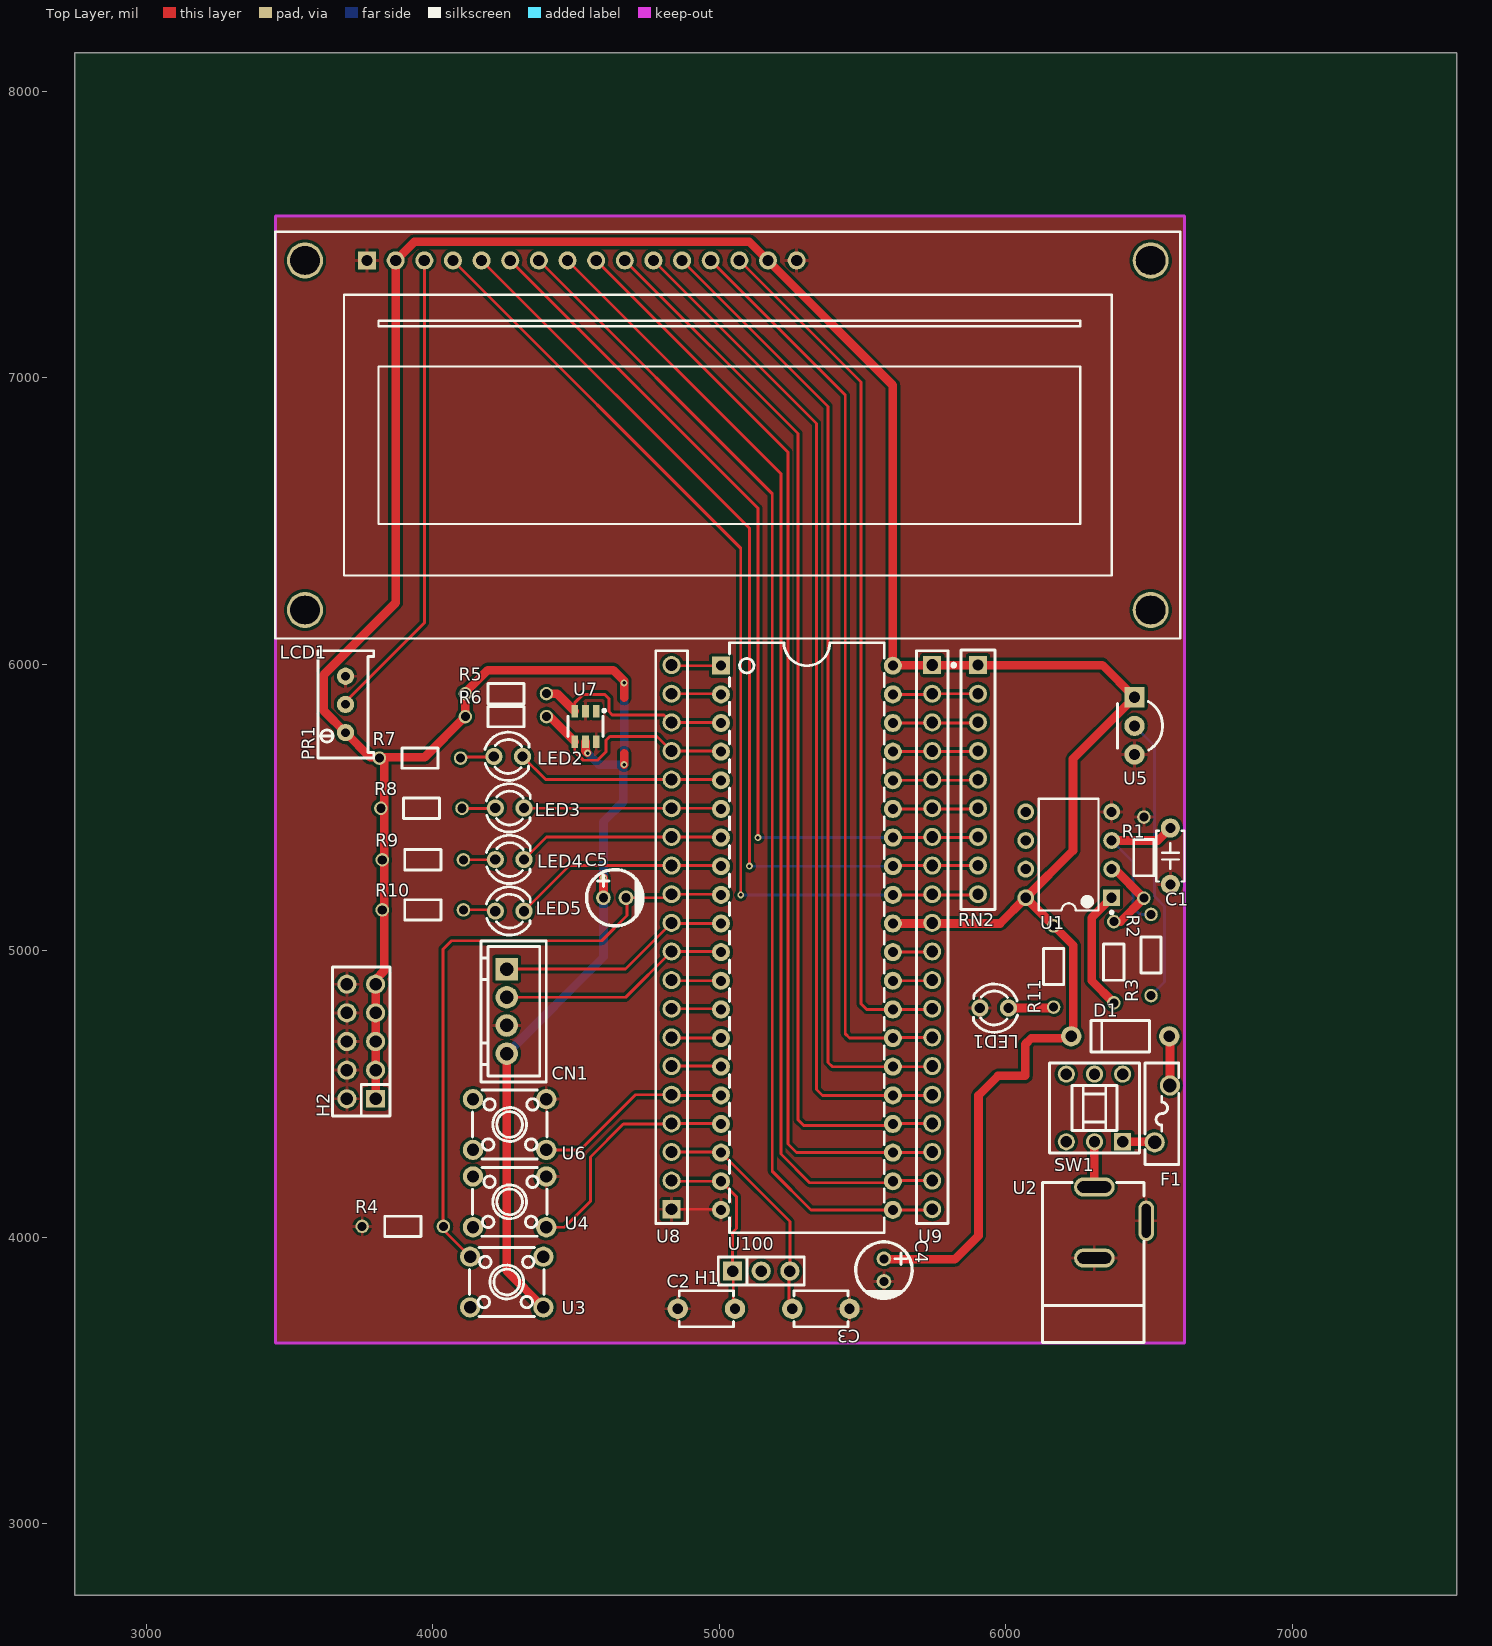
[diagram p0: Top Layer view]
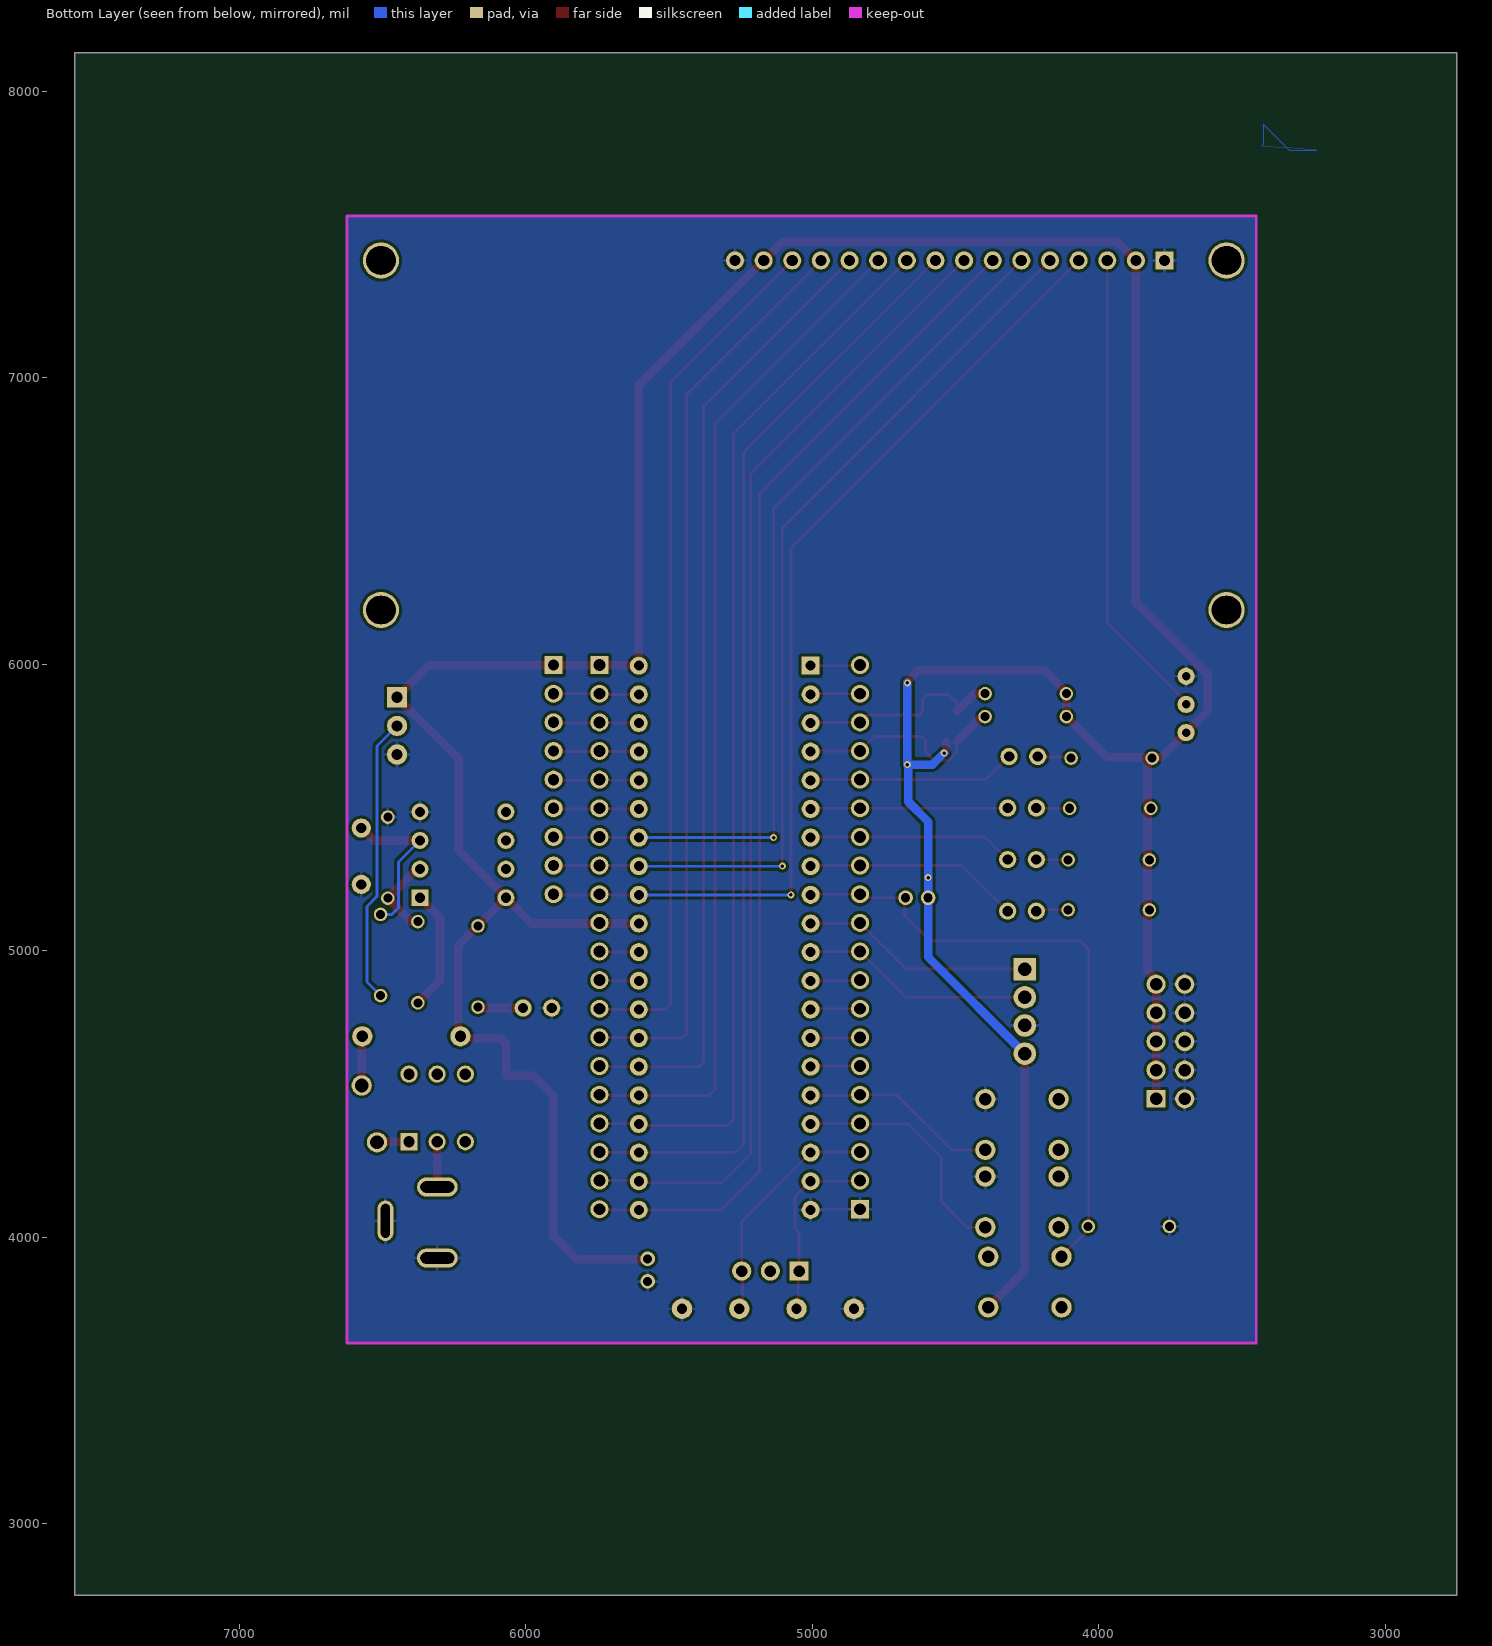
[diagram p1: Bottom Layer view, seen from below]
# Altium PCB MISC75226.pcbdoc
Units mil, origin at the board's own origin, x right, y up, seen from the top; angles counter-clockwise.
Board outline 4825 x 5385 mil, 2 copper layers (Top Layer, Bottom Layer), stack 2.757 mil thick; 40 components, 54 nets, 213 pads, 7 vias.

## Layer stack, top to bottom
Top Solder Mask Layer: solder mask 0.394, Dk 3.3
Top Layer: signal copper 1.379
Bottom Layer: signal copper 1.378
Bottom Solder Mask Layer: solder mask 0.394, Dk 3.3

## Board outline
7575,2750 2750,2750 2750,8135 7575,8135

## Design rules (kind name [scope] priority, off if disabled: settings)
BoardOutlineClearance Default_1 [All] p2: genericclearance=4 ignorepadtopadclearanceinfootprint=FALSE except(0: Arc-SplitContinuation Track-SplitContinuation SMDPad-SplitContinuation THPad-SplitContinuation Via-SplitContinuation Fill-SplitContinuation Region-SplitContinuation Poly-SplitContinuation Text-SplitContinuation Hole-SplitContinuation; 6: Arc-OutlineEdge Track-OutlineEdge SMDPad-OutlineEdge THPad-OutlineEdge Via-OutlineEdge Fill-OutlineEdge Region-OutlineEdge Poly-OutlineEdge Text-OutlineEdge Hole-OutlineEdge SMDPad-CutoutEdge THPad-CutoutEdge Via-CutoutEdge Fill-CutoutEdge Region-CutoutEdge Text-CutoutEdge; 6.9: Hole-CutoutEdge; 10: Poly-CutoutEdge; 11.8: Arc-CutoutEdge Track-CutoutEdge)
Clearance Default [All] p1: gap=4 ignorepadtopadclearanceinfootprint=FALSE except(6: SMDPad-Track SMDPad-SMDPad THPad-Track SMDPad-THPad THPad-THPad Track-Via SMDPad-Via THPad-Via Via-Via Fill-Track Region-Track Fill-SMDPad Region-SMDPad Fill-THPad Region-THPad Fill-Via Region-Via Fill-Fill Fill-Region Region-Region Arc-Track Arc-SMDPad Arc-THPad Arc-Via Fill-Arc Region-Arc Arc-Arc Text-Track SMDPad-Text Text-THPad Text-Via Fill-Text Region-Text Arc-Text Text-Text; 6.9: Hole-Track Hole-SMDPad Hole-THPad Hole-Via Fill-Hole Region-Hole Hole-Arc Hole-Text; 10: Poly-Track Poly-SMDPad Poly-THPad Poly-Via Poly-Fill Poly-Region Poly-Poly Poly-Arc Poly-Text Poly-Hole)
DiffPairsRouting differentialPair [All] p1: maxlimit=6 minlimit=5 mostfreqgap=6 toplayer_minwidth=5 toplayer_prefwidth=100 toplayer_maxwidth=100 toplayer_mingap=5 toplayer_prefgap=6 toplayer_maxgap=6 bottomlayer_minwidth=5 bottomlayer_prefwidth=100 bottomlayer_maxwidth=100 bottomlayer_mingap=5 bottomlayer_prefgap=6 bottomlayer_maxgap=6 maxuncoupledlength=10
HoleToHoleClearance otherClearance [All] p1: gap=11.8 allowstackedmicrovias=TRUE
Length netLength [All] p1: minlimit=0 maxlimit=0
MatchedLengths netLengthTolerance [All] p1: tolerance=1000
PasteMaskExpansion pasteMaskExpansion [All] p1: expansion=0
PlaneConnect innerPlane [All] p1: planeconnectstyle=Relief reliefexpansion=20 reliefentries=4 reliefconductorwidth=10 reliefairgap=10
PolygonConnect copperRegion [All] p1: connectstyle=Relief reliefconductorwidth=10 reliefentries=4 polygonreliefangle="90 Angle" airgapwidth=10 via.connectstyle=Relief via.reliefconductorwidth=10 via.reliefentries=4 via.polygonreliefangle="90 Angle" via.airgapwidth=10
RoutingVias Default_3 [All] p1: holewidth=12 width=24 viastyle="Through Hole" minholewidth=12 minwidth=24 maxholewidth=1181 maxwidth=1969
SolderMaskExpansion Common [IsVia] p1: expansion=-1000 istentingtop=TRUE
SolderMaskExpansion Common [All] p2: expansion=2 istentingtop=FALSE
Width Default_2 [All] p1: maxlimit=1000 minlimit=10 preferedwidth=10

## Components (designator, comment, footprint, x,y, rotation, side; value= is the part's Value field where it differs from the comment)
C1 "10nF" CAP-TH_L4.5-W2.5-P5.00-D0.5 6575,5330 r90 top
C2 "22pF" CAP-TH_L4.8-W3.2-P5.08-D0.5 4955,3750 r0 top
C3 "22pF" CAP-TH_L4.8-W3.2-P5.08-D0.5 5355,3750 r180 top
C4 "10uF" CAP-TH_BD5.0-P2.00-D0.8-FD-10UF50VC110GL 5575,3885 r270 top
C5 "10uF" CAP-TH_BD5.0-P2.00-D0.8-FD-10UF50VC110GL 4635,5185 r0 top
CN1 "HEADER 4" CONN-TH_XH-4A 4258.04,4788.24 r270 top
D1 "1N4007" DO-41_BD2.4-L4.7-P8.70-D0.9-RD 6400.04,4701.07 r0 top
F1 "JK60-050" FUSE-TH_L8.9-W3.0-P5.10-D0.6-S1.20 6545.04,4431.07 r90 top
H1 "PZ254V-11-03P_C2937625" HDR-TH_3P-P2.54-V-M_PZ254V-11-03P 5146.55,3881.61 r0 top
H2 "" HDR-TH_10P-P2.54-V-F-R2-C5-S2.54 3749.9,4683.05 r90 top
LCD1 "HS1602A" LCD1602 5030,6800 r0 top
LED1 "" LED_TH-3mm 5960,4800 r180 top
LED2 "HL-304S9AD" LED-TH_BD3.0-P2.54-FD 4263.04,5678.24 r0 top
LED3 "HL-304S9AD" LED-TH_BD3.0-P2.54-FD 4268.04,5498.24 r0 top
LED4 "HL-304S9AD" LED-TH_BD3.0-P2.54-FD 4268.04,5318.24 r0 top
LED5 "HL-304S9AD" LED-TH_BD3.0-P2.54-FD 4268.04,5138.24 r0 top
PR1 "10kΩ" R_3296 3690,5860 r90 top
R1 "10kΩ" Res_1/8W 6480,5325 r270 top
R2 "10kΩ" Res_1/8W 6375,4960 r270 top
R3 "10kΩ" Res_1/8W 6510,4985 r90 top
R4 "10kΩ" Res_1/8W 3895,4035 r0 top
R5 "10kΩ" Res_1/8W 4255,5895 r0 top
R6 "10kΩ" Res_1/8W 4255,5815 r0 top
R7 "1kΩ" Res_1/8W 3955,5670 r0 top
R8 "1kΩ" Res_1/8W 3960,5495 r0 top
R9 "1kΩ" Res_1/8W 3965,5315 r0 top
R10 "1kΩ" Res_1/8W 3965,5140 r0 top
R11 "1kΩ" Res_1/8W 6170,4945 r90 top
RN2 "10K" RES-ARRAY-TH_9P-P2.54-D1.0 5903.48,5597.32 r270 top
SW1 "HX 8-8 ZS" SW-TH_6P-L8.0-W8.0-P2.50-TL 6310.04,4451.07 r180 top
U1 "LM358AN" DIP-8_L9.8-W6.6-P2.54-LS7.6-BL 6220,5335 r90 top
U2 "DC005-2.5" DC-IN-TH_DC005-2.5MM 6400.04,4051.07 r90 top
U3 "TC-00104FS-075E" KEY-TH_4P-L6.0-W6.0-P4.50-LS6.5 4258.04,3843.24 r0 top
U4 "TC-00104FS-075E" KEY-TH_4P-L6.0-W6.0-P4.50-LS6.5 4268.04,4123.24 r180 top
U5 "LM35DZ/NOPB" TO-92-3_L4.8-W3.7-P2.54-L 6450,5785 r270 top
U6 "TC-00104FS-075E" KEY-TH_4P-L6.0-W6.0-P4.50-LS6.5 4268.04,4393.24 r180 top
U7 "ADS1110A1IDBVR" SOT-23-6_L2.9-W1.6-P0.95-LS2.8-BR 4533.04,5783.24 r90 top
U8 "[Plugin] 2.54MM 1*20P straight female header-H5.0" HDR-TH_20P-P2.54_C9900009338 4833.48,5047.32 r90 top
U9 "[Plugin] 2.54MM 1*20P straight female header-H5.0" HDR-TH_20P-P2.54_C9900009338 5743.48,5047.32 r270 top
U100 "STC89C52RC-40I" DIP-40_L52.0-W13.7-P2.54-LS15.2-BL 5305.96,5045.14 r270 top

## Footprints (in the part's own frame and the unit in brackets; to place one, negate y for a bottom-side part, rotate by r counter-clockwise, add the part's x,y. Pads: shape width x height; smd on the part's side, far side on the other; paste and mask are expansions set on the pad)
CAP-TH_BD5.0-P2.00-D0.8-FD-10UF50VC110GL [mm]
  round 1.3 hole 0.8: 1(-1,0) 2(1,0)
  silkscreen extent -2.5,-2.5 2.5,2.5
CAP-TH_L4.5-W2.5-P5.00-D0.5 [mm]
  round 1.7 hole 0.9 paste+0 mask+0.05: 1(-2.5,0) 2(2.5,0)
  silkscreen extent -2.25,-1.25 2.25,1.25
CAP-TH_L4.8-W3.2-P5.08-D0.5 [mm]
  round 1.8 hole 0.9: 1(-2.54,0) 2(2.54,0)
  silkscreen extent -2.4,-1.6 2.4,1.6
CONN-TH_XH-4A [mm]
  rect 2x2 hole 1.2 paste+0 mask+0.051: 1(-3.75,0)
  round 2 hole 1.2 paste+0 mask+0.051: 2(-1.25,0) 3(1.25,0) 4(3.75,0)
  silkscreen extent -6.25,-2.3 6.25,3.5
DC-IN-TH_DC005-2.5MM [mm]
  oval 3.6x1.4 hole 0.8 slot 3 at 0 deg copper offset 0,0 paste+0 mask+0.05: 2(0.15,-2.3)
  oval 1.7x3.6 hole 1 slot 3 at 90 deg copper offset 0,0 paste+0 mask+0.05: 3(-3.15,2.3)
  oval 1.7x3.6 hole 1 slot 3 at 90 deg paste+0 mask+0.05: 4(3.15,2.3)
  silkscreen extent -10.65,-2.1 3.55,6.9
DIP-8_L9.8-W6.6-P2.54-LS7.6-BL [mm]
  rect 1.5x1.5 hole 0.9 paste+0 mask+0.051: 1(-3.81,-3.81)
  round 1.5 hole 0.9 paste+0 mask+0.051: 2(-1.27,-3.81) 3(1.27,-3.81) 4(3.81,-3.81) 5(3.81,3.81) 6(1.27,3.81) 7(-1.27,3.81) 8(-3.81,3.81)
  silkscreen extent -5.23,-3.93 4.96,2.65
DIP-40_L52.0-W13.7-P2.54-LS15.2-BL [mil]
  rect 63x63 hole 35 paste+0 mask+2: 1(-950,-300)
  round 63 hole 35 paste+0 mask+2: 2(-850,-300) 3(-750,-300) 4(-650,-300) 5(-550,-300) 6(-450,-300) 7(-350,-300) 8(-250,-300) 9(-150,-300) 10(-50,-300) 11(50,-300) 12(150,-300) 13(250,-300) 14(350,-300) 15(450,-300) 16(550,-300) 17(650,-300) 18(750,-300) 19(850,-300) 20(950,-300) 21(950,300) 22(850,300) 23(750,300) 24(650,300) 25(550,300) 26(450,300) 27(350,300) 28(250,300) 29(150,300) 30(50,300) 31(-50,300) 32(-150,300) 33(-250,300) 34(-350,300) 35(-450,300) 36(-550,300) 37(-650,300) 38(-750,300) 39(-850,300) 40(-950,300)
  silkscreen extent -1030,-270 1030,270
DO-41_BD2.4-L4.7-P8.70-D0.9-RD [mm]
  round 1.8 hole 1 paste+0 mask+0.051: 1(-4.35,0) 2(4.35,0)
  silkscreen extent -2.6,-1.4 2.6,1.4
FUSE-TH_L8.9-W3.0-P5.10-D0.6-S1.20 [mm]
  round 1.8 hole 1.2 paste+0 mask+0.051: 1(-2.54,0.635) 2(2.499,-0.727)
  silkscreen extent -4.5,-1.5 4.5,1.5
HDR-TH_3P-P2.54-V-M_PZ254V-11-03P [mm]
  rect 1.7x1.7 hole 1.02 paste+0 mask+0.051: 1(-2.54,0)
  round 1.7 hole 1.02 paste+0 mask+0.051: 2(0,0) 3(2.54,0)
  silkscreen extent -3.81,-1.25 3.81,1.25
HDR-TH_10P-P2.54-V-F-R2-C5-S2.54 [mm]
  rect 1.575x1.7 hole 1.1: 1(-5.08,-1.27)
  round 1.7 hole 1.1: 2(-5.08,1.27) 3(-2.54,-1.27) 4(-2.54,1.27) 5(0,-1.27) 6(0,1.27) 7(2.54,-1.27) 8(2.54,1.27) 9(5.08,-1.27) 10(5.08,1.27)
  silkscreen extent -6.6,-2.54 6.6,2.54
HDR-TH_20P-P2.54_C9900009338 [mm]
  rect 1.6x1.6 hole 1.05 paste+0 mask+0.051: 1(-24.13,0)
  round 1.6 hole 1.05 paste+0 mask+0.051: 2(-21.59,0) 3(-19.05,0) 4(-16.51,0) 5(-13.97,0) 6(-11.43,0) 7(-8.89,0) 8(-6.35,0) 9(-3.81,0) 10(-1.27,0) 11(1.27,0) 12(3.81,0) 13(6.35,0) 14(8.89,0) 15(11.43,0) 16(13.97,0) 17(16.51,0) 18(19.05,0) 19(21.59,0) 20(24.13,0)
  silkscreen extent -25.4,-1.4 25.4,1.4
KEY-TH_4P-L6.0-W6.0-P4.50-LS6.5 [mm]
  round 1.8 hole 1.1 paste+0 mask+0.051: 1(-3.251,-2.25) 2(3.251,-2.25) 3(3.251,2.25) 4(-3.251,2.25)
  silkscreen extent -3.3,-3.05 3.3,3.05
LCD1602 [mm]
  round 3.2 hole 2.5 slot 2.625 at 0 deg paste+0 mask+0.051: 0(-37.5,-15.5) 0(-37.5,15.5) 0(37.5,-15.5) 0(37.5,15.5)
  rect 1.6x1.6 hole 1 paste+0 mask+0.051: 1(-32,15.5)
  round 1.6 hole 1 paste+0 mask+0.051: 2(-29.46,15.5) 3(-26.92,15.5) 4(-24.38,15.5) 5(-21.84,15.5) 6(-19.3,15.5) 7(-16.76,15.5) 8(-14.22,15.5) 9(-11.68,15.5) 10(-9.14,15.5) 11(-6.6,15.5) 12(-4.06,15.5) 13(-1.52,15.5) 14(1.02,15.5) 15(3.56,15.5) 16(6.1,15.5)
  silkscreen extent -40.13,-18.03 40.13,18.03
LED-TH_BD3.0-P2.54-FD [mil]
  round 60 hole 36 paste+0 mask+1.97: 1(-50,0) 2(50,0)
  silkscreen extent -81,-84 72,85
LED_TH-3mm [mil]
  round 60 hole 36 paste+0 mask+2: 1(-50,0) 2(50,0)
  silkscreen extent -81,-84 72,85
R_3296 [mil]
  round 60 hole 30 paste+0 mask+2: 1(-98.4,-5) 2(0,-5) 3(98.4,-5)
  silkscreen extent -187,-103 187,92
RES-ARRAY-TH_9P-P2.54-D1.0 [mm]
  rect 1.6x1.6 hole 1 paste+0 mask+0.051: 1(-10.16,0)
  round 1.6 hole 1 paste+0 mask+0.051: 2(-7.62,0) 3(-5.08,0) 4(-2.54,0) 5(0,0) 6(2.54,0) 7(5.08,0) 8(7.62,0) 9(10.16,0)
  silkscreen extent -11.5,-2.31 11.5,1.5
Res_1/8W [mil]
  round 47.2 hole 31.5 paste+0 mask+2: 1(-141.7,2.48) 2(141.7,2.48)
  silkscreen extent -63,-33 63,38
SOT-23-6_L2.9-W1.6-P0.95-LS2.8-BR [mm]
  rect 1.1x0.6 smd paste+0 mask+0.051: 1(1.35,-0.95) 2(1.35,0) 3(1.35,0.95) 4(-1.35,0.95) 5(-1.35,0) 6(-1.35,-0.95)
  silkscreen extent -0.9,-1.78 1.52,1.55
SW-TH_6P-L8.0-W8.0-P2.50-TL [mil]
  rect 60x60 hole 39.37 paste+0 mask+2: 1(-98.42,118.11)
  round 60 hole 39.37 paste+0 mask+2: 2(0.01,118.11) 3(98.43,118.11) 4(-98.42,-118.11) 5(0.01,-118.11) 6(98.43,-118.11)
  silkscreen extent -157,-157 157,157
TO-92-3_L4.8-W3.7-P2.54-L [mm]
  rect 1.8x1.8 hole 1 paste+0 mask+0.051: 1(-2.54,0)
  round 1.8 hole 1 paste+0 mask+0.051: 2(0,0) 3(2.54,0)
  silkscreen extent -2.17,-1.5 2.14,2.48

## Via types
v1: diameter 24.41, hole 12.2, Top Layer to Bottom Layer, 7 vias

## Nets (pads, with @x,y where several pads share a name; then routed paths per layer and width w, separated by ;. In a path a pad name is that pad's centre, name@x,y a point inside that pad or via, vN(x,y) a via of type N, cw(c..) or ccw(c..) an arc to the next point about the centre after c; other vN are vias at no path point)
$2N1: SW1.2 U2.4 | length 157.9
  Top Layer w30: U2.4 SW1.2
$2N3: F1.1 SW1.1 | length 112.4
  Top Layer w30: SW1.1 6518.15,4332.96 F1.1
$2N4: D1.2 F1.2 | length 176.1
  Top Layer w10: F1.2@6568.66,4529.47 F1.2@6571.16,4531.97
  Top Layer w30: D1.2 6573.66,4698.71 F1.2
$2N6: LED1.1 R11.1 | length 158.9
  Top Layer w30: LED1.1 6164.22,4800 R11.1
$2N21: H1.2
$2N22: C1.2 R3.2 U1.3 | length 561.2
  Top Layer w30: U1.3 6531.57,5385 C1.2
  Bottom Layer w10: U1.3 6445,5310 6445,5150 6468.3,5126.7 R3.2
$2N23: R1.2 R2.1 U1.2 | length 293.4
  Top Layer w30: U1.2 6380.78,5285 R1.2 6400.88,5101.7 R2.1
$2N29: LED2.1 R7.2 | length 111.3
  Top Layer w10: R7.2@4102.7,5675.89 4210.69,5675.89 LED2.1
$2N31: LED3.1 R8.2 | length 116
  Top Layer w10: R8.2@4102.7,5496.68 4216.48,5496.68 LED3.1
$2N32: LED4.1 R9.2 | length 115.3
  Top Layer w10: R9.2@4102.7,5317.5 LED4.1
$2N33: LED5.1 R10.2 | length 117.4
  Top Layer w10: R10.2@4102.7,5143.24 4213.04,5143.24 LED5.1
ALE: U9.11 U100.30 | length 138.4
  Top Layer w10: U100.30 5741.3,4995.14 U9.11
GND: C1.1 C2.1 C3.1 C4.2 CN1.3 H2.2 H2.4 H2.6 H2.8 H2.10 LCD1.1 LCD1.16 LED1.2 PR1.3 R1.1 R4.1 U1.4 U2.2 U2.3 U4.1 U5.3 U6.1 U7.2 U7.6 U8.1 U100.20 | length 173.4
  Top Layer w10: U8.1 5003.78,4097.32 U100.20
P0.0: RN2.2 U9.2 U100.39 | length 298.4
  Top Layer w10: U100.39 5741.3,5895.14 U9.2 RN2.2
P0.1: RN2.3 U9.3 U100.38 | length 298.4
  Top Layer w10: U100.38 5901.3,5795.14 RN2.3
P0.2: RN2.4 U9.4 U100.37 | length 298.4
  Top Layer w10: U100.37 5901.3,5695.14 RN2.4
P0.3: RN2.5 U9.5 U100.36 | length 298.4
  Top Layer w10: U100.36 5901.3,5595.14 RN2.5
P0.4: RN2.6 U9.6 U100.35 | length 298.4
  Top Layer w10: U100.35 5901.3,5495.14 RN2.6
P0.5: LCD1.6 RN2.7 U9.7 U100.34 | length 3142.9
  Top Layer w10: LCD1.6 4270.16,7409.84 5065,6615 5135,6545 v1(5135,5395) ; U100.34 5901.3,5395.14 RN2.7
  Bottom Layer w10: v1(5135,5395) U100.34
P0.6: LCD1.5 RN2.8 U9.8 U100.33 | length 3301.7
  Top Layer w10: LCD1.5 5105,6475.4 v1(5105,5295.14) ; U100.33 5608.14,5297.32 U9.8 RN2.8
  Bottom Layer w10: v1(5105,5295.14) U100.33
P0.7: LCD1.4 RN2.9 U9.9 U100.32 | length 3460.7
  Top Layer w10: LCD1.4 5075,6405.4 v1(5075,5195.14) ; U100.32 5901.3,5195.14 RN2.9
  Bottom Layer w10: v1(5075,5195.14) U100.32
P1.0: U8.20 U100.1 | length 173.4
  Top Layer w10: U8.20 4835.66,5995.14 U100.1
P1.1: U8.19 U100.2 | length 173.4
  Top Layer w10: U8.19 5003.78,5897.32 U100.2
P1.2: R5.2 U7.3 U8.18 U100.3 | length 743.7
  Top Layer w10: U7.3 4495.64,5865.64 4525,5895 4600,5895 4615,5880 4615,5835 4626.42,5823.58 4807.22,5823.58 U8.18 5003.78,5797.32 U100.3
  Top Layer w30: R5.2 4434.55,5897.48 U7.3
P1.3: R6.2 U7.4 U8.17 U100.4 | length 773
  Top Layer w10: U7.4 4495.64,5694.36 4525,5665 4575,5665 4605,5695 4605,5735 4617.9,5747.9 4782.9,5747.9 U8.17 5003.78,5697.32 U100.4
  Top Layer w30: R6.2 4408.25,5817.48 U7.4
P1.4: LED2.2 U8.16 U100.5 | length 727.3
  Top Layer w10: LED2.2 4393.96,5597.32 U8.16 5003.78,5597.32 U100.5
P1.5: LED3.2 U8.15 U100.6 | length 688.9
  Top Layer w10: LED3.2 U8.15 5003.78,5497.32 U100.6
P1.6: LED4.2 U8.14 U100.7 | length 721.6
  Top Layer w10: LED4.2 4397.12,5397.32 U8.14 5003.78,5397.32 U100.7
P1.7: LED5.2 U8.13 U100.8 | length 754.7
  Top Layer w10: LED5.2 4477.12,5297.32 U8.13 5003.78,5297.32 U100.8
P2.0: LCD1.7 U9.20 U100.21 | length 4133
  Top Layer w10: LCD1.7 5185,6595.4 5185,4230 5319.9,4095.1 U100.21 ; U100.21 5741.3,4095.14 U9.20
P2.1: LCD1.8 U9.19 U100.22 | length 4001.6
  Top Layer w10: LCD1.8 5215,6665.4 5215,4290 5315,4190 5600.8,4190 U100.22 ; U100.22 5608.14,4197.32 U9.19
P2.2: LCD1.9 U9.18 U100.23 | length 3879.4
  Top Layer w10: LCD1.9 5240,6740.4 5240,4325 5269.9,4295.1 U100.23 ; U100.23 5741.3,4295.14 U9.18
P2.3: LCD1.10 U9.17 U100.24 | length 3730.5
  Top Layer w10: LCD1.10 5275,6805.4 5275,4410 5295,4390 5600.8,4390 U100.24 ; U100.24 5608.14,4397.32 U9.17
P2.4: LCD1.11 U9.16 U100.25 | length 3543.9
  Top Layer w10: LCD1.11 5340,6840.4 5340,4515 5359.9,4495.1 U100.25 ; U100.25 5741.3,4495.14 U9.16
P2.5: LCD1.12 U9.15 U100.26 | length 3382
  Top Layer w10: LCD1.12 5380,6900.4 5380,4610 5395,4595 U100.26 ; U100.26 5741.3,4595.14 U9.15
P2.6: LCD1.13 U9.14 U100.27 | length 3205.4
  Top Layer w10: LCD1.13 5440,6940.4 5440,4710 5454.9,4695.1 U100.27 ; U100.27 5608.14,4697.32 U9.14
P2.7: LCD1.14 U9.13 U100.28 | length 3028.8
  Top Layer w10: LCD1.14 5495,6985.4 5495,4815 5514.9,4795.1 U100.28 ; U100.28 5741.3,4795.14 U9.13
P3.2: U8.9 U100.12 | length 173.4
  Top Layer w10: U8.9 4835.66,4895.14 U100.12
P3.3: U8.8 U100.13 | length 173.4
  Top Layer w10: U8.8 5003.78,4797.32 U100.13
P3.4: U8.7 U100.14 | length 173.4
  Top Layer w10: U8.7 4835.66,4695.14 U100.14
P3.5: U8.6 U100.15 | length 173.4
  Top Layer w10: U8.6 5003.78,4597.32 U100.15
P3.6: U6.4 U8.5 U100.16 | length 690.6
  Top Layer w10: U6.4 4514.64,4304.64 4707.32,4497.32 U8.5 4835.66,4495.14 U100.16
P3.7: U4.4 U8.4 U100.17 | length 851.8
  Top Layer w10: U4.4 4459.64,4034.64 4550,4125 4550,4280 4665,4395 4831.16,4395 U8.4 5003.78,4397.32 U100.17
PSEN: U9.12 U100.29 | length 138.4
  Top Layer w10: U100.29 5741.3,4895.14 U9.12
RST: C5.2 R4.2 U3.4 U8.12 U100.9 | length 2220.1
  Top Layer w10: U3.4 4035,4026.88 4035,5005 4065,5035 4589.46,5035 4677.7,5123.24 C5.2@4677.7,5185 ; C5.2@4677.7,5196.84 C5.2@4677.7,5188.33 ; U100.9 5003.78,5197.32 U8.12 4821.16,5185 C5.2@4677.7,5185 ; C5.2@4677.7,5185 C5.2 C5.2@4677.7,5188.33 ; C5.2@4677.7,5185 C5.2@4677.7,5188.33
RXD_TTL: CN1.1 U8.11 U100.10 | length 815.7
  Top Layer w10: CN1.1 4672.04,4935.88 U8.11 4835.66,5095.14 U100.10
S$6580: 
TXD_TTL: CN1.2 U8.10 U100.11 | length 815
  Top Layer w10: CN1.2 4673.61,4837.45 U8.10 5003.78,4997.32 U100.11
U6.1: R2.2 U1.1 | length 427.8
  Top Layer w30: U1.1 6300,5115 6300,4895.78 R2.2
VCC: C4.1 C5.1 CN1.4 D1.1 H2.1 H2.3 H2.5 H2.7 H2.9 LCD1.2 LCD1.15 PR1.1 R5.1 R6.1 R7.1 R8.1 R9.1 R10.1 R11.2 RN2.1 U1.8 U3.2 U5.1 U7.5 U9.1 U9.10 U100.31 U100.40 | length 13956.6
  Top Layer w10: U9.10@5741.3,5095.14 U9.10
  Top Layer w30: H2.1 H2.3 H2.5 H2.7 H2.9 3799.9,4899.76 3829.9,4929.76 3829.9,5669.9 R7.1@3835.89,5675.89 ; R5.1@4111.15,5899.63 4191.52,5980 4630,5980 4668.04,5941.96 4668.04,5882.9 ; R5.1 R6.1 3971.72,5675.89 R7.1@3835.89,5675.89 ; CN1.4 4258.04,3882.64 U3.2 ; U7.5 4533.04,5696.96 v1@4538.93,5691.07 ; C5.1 4595.63,5254.83 v1(4595.8,5255) ; v1(4668.04,5650) 4668.04,5688.58 ; C4.1 5577.05,3922.32 5822.32,3922.32 5905,4005 5905,4495 5972.82,4562.82 6068.73,4562.82 6068.73,4673.79 6089.95,4695 6192.04,4695 ; U100.31 5741.3,5095.14 5980.14,5095.14 U1.8 ; 6236.65,4737.2 6236.65,5018.35 U1.8 ; R7.1@3835.89,5675.89 3780.71,5675.89 PR1.1 3618.98,5837.62 3618.98,5963.98 3870.16,6215.16 LCD1.2 3934.92,7475 5105.4,7475 LCD1.15 5605.96,6974.44 U100.40 5608.14,5997.32 U9.1 RN2.1 6337.68,5997.32 U5.1 6235,5670 6235,5350 U1.8
  Bottom Layer w30: CN1.4 4595.8,4978.36 v1(4595.8,5255) 4595.8,5450.8 4665,5520 4665,5646.96 v1(4668.04,5650) ; v1(4540,5690) 4580,5650 v1(4668.04,5650) ; v1(4668.04,5935) v1(4668.04,5650)
VO: LCD1.3 PR1.2 | length 1662.1
  Top Layer w10: PR1.2@3690.01,5864.21 3970.16,6144.37 LCD1.3
VOUT: R3.1 U5.2 | length 1004.9
  Bottom Layer w10: U5.2 6520,5715 6520,5190 6555,5155 6555,4890.78 R3.1
XTAL1: C2.2 H1.1 U8.2 U100.19 | length 620.9
  Top Layer w10: U8.2 4835.66,4195.14 U100.19 5060,4141.1 5060,4030 5046.55,4016.55 H1.1 5048.99,3879.17 C2.2@5048.99,3776.61
XTAL2: C3.2 H1.3 U8.3 U100.18 | length 792.6
  Top Layer w10: U8.3 5003.78,4297.32 U100.18 5246.55,4054.55 H1.3 5244.11,3879.17 C3.2@5244.11,3776.61
pads on no net: LCD1.0 SW1.3 SW1.4 SW1.5 SW1.6 U1.5 U1.6 U1.7 U3.1 U3.3 U4.2 U4.3 U6.2 U6.3 U7.1

## Polygon pours and split planes (outlines as drawn)
GND on Top Layer (solid, remove dead copper, pour order 2): 3220,7615 6850,7615 7040,7425 7040,3840 6490,3290 3515,3290 3050,3755 3050,7440 3180,7570 3180,7605 3220,7645
GND on Bottom Layer (solid, remove dead copper, pour order 6): 3460,3000 3000,3460 3000,7460 3335,7795 6985,7795 7325,7455 7325,3215 7110,3000
GND on Bottom Layer (solid, remove dead copper, pour order 6): 3335,7795 3240,7795 3343.14,7803.14
GND on Bottom Layer (solid, remove dead copper, pour order 6): 3343.14,7803.14 3425,7885 3425,7815 3430,7810

## Keep-outs
Board Outline Layer:
  lines w10 net S$6580: 3450,3630 6625,3630 6625,7565 3450,7565 3450,3630